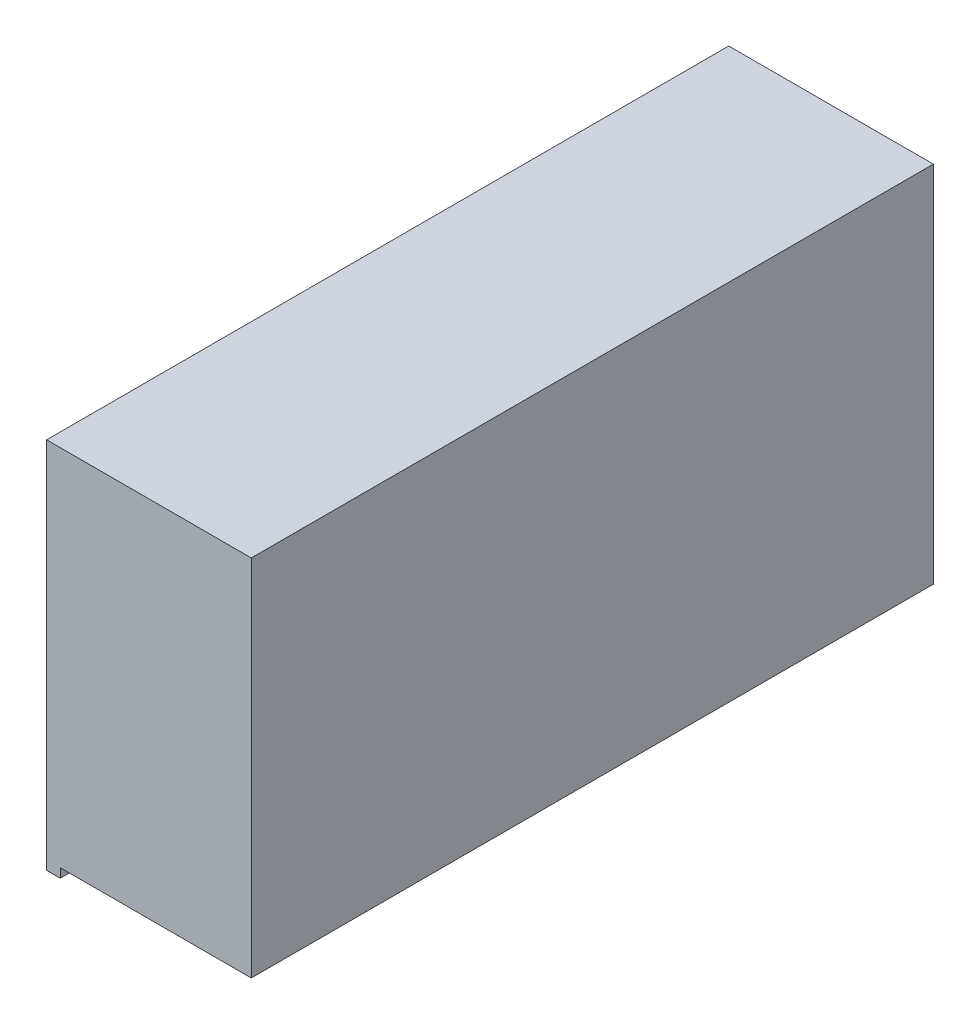
from build123d import *

# Parameters (mm, degrees)
EXTRUDE_1_DEPTH = 75


with BuildPart() as part:
    # 草图1 → 凸台-拉伸1 (new, symmetric)
    with BuildSketch(Plane.XY):
        Polygon((0, 0), (0, 82), (45, 82), (45, 2), (3, 2), (3, 0), align=None)
    extrude(amount=EXTRUDE_1_DEPTH, both=True)


solid = part.part
